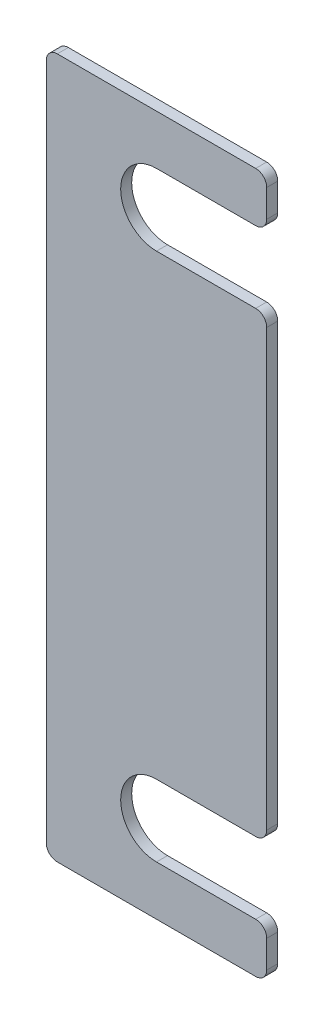
SolidWorks part; units mm, degrees
ref_plane "前视基准面" through (0, 0, 0) normal (0, 0, 1) x (1, 0, 0)
ref_plane "上视基准面" through (0, 0, 0) normal (0, 1, 0) x (1, 0, 0)
ref_plane "右视基准面" through (0, 0, 0) normal (1, 0, 0) x (0, 0, -1)
sketch "草图1" plane through (0, 0, 0) normal (0, 0, 1) x (1, 0, 0)
  line L1 (20, -63.5) -> (-20, -63.5)
  line L2 (20, -63.5) -> (20, 63.5)
  line L3 (20, 63.5) -> (-20, 63.5)
  line L4 (-20, -63.5) -> (-20, 63.5)
  line L5 (20, -63.5) -> (-20, 63.5) construction
  line L6 (20, 63.5) -> (-20, -63.5) construction
  point P0 (0, 0)
  dimension "D1" = 40
  dimension "D2" = 127
extrude "凸台-拉伸1" add sketch "草图1" along normal blind 2
sketch "草图2" plane through (0, 0, 2) normal (0, 0, 1) x (1, 0, 0)
  line L2 (0, -48) -> (0, 48) construction
  circle A2 centre (0, 48) radius 6.5
  circle A3 centre (0, -48) radius 6.5
  point P0 (0, 0)
  dimension "D3" = 13
  dimension "D1" = 96
extrude "切除-拉伸1" cut sketch "草图2" against normal blind 3
sketch "草图4" plane through (0, 0, 2) normal (0, 0, 1) x (1, 0, 0)
  line L0 (20, -63.5) -> (20, 63.5) construction
  line L17 (0, 41.5) -> (20, 41.5)
  line L18 (0, 41.5) -> (0, 54.5)
  line L19 (0, 54.5) -> (20, 54.5)
  line L20 (20, 41.5) -> (20, 54.5)
  line L22 (0, -41.5) -> (20, -41.5)
  line L23 (0, -41.5) -> (0, -54.5)
  line L24 (0, -54.5) -> (20, -54.5)
  line L25 (20, -41.5) -> (20, -54.5)
  circle A4 centre (0, 48) radius 6.5 construction
  circle A5 centre (0, -48) radius 6.5 construction
extrude "切除-拉伸4" cut sketch "草图4" against normal blind 10
fillet "圆角2" radius 2 8 edges at (-20, -63.5, 1) (-20, 63.5, 1) (20, -63.5, 1) (20, 63.5, 1) (20, -54.5, 1) (20, -41.5, 1) (20, 41.5, 1) (20, 54.5, 1)
